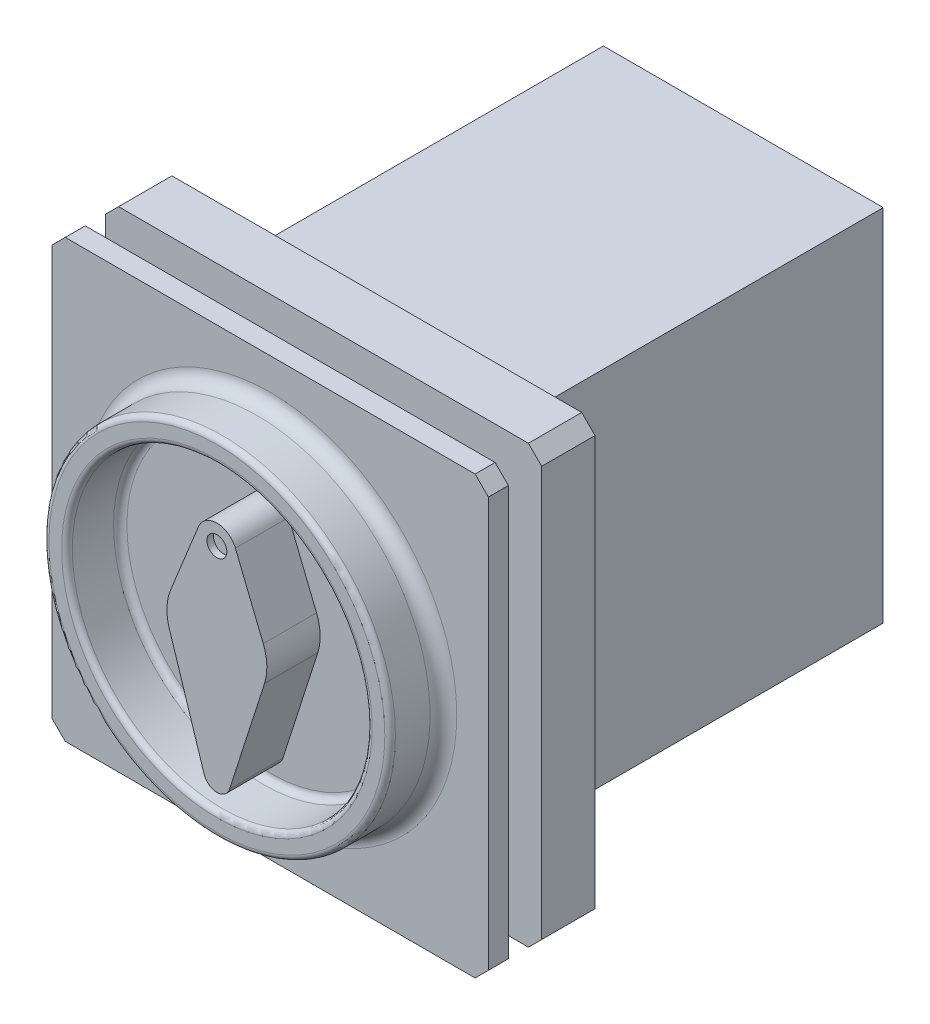
from build123d import *

# Parameters (mm, degrees)
SKETCH_1_W             = 42
SKETCH_1_H             = 54
EXTRUDE_1_DEPTH        = 55
SKETCH_5_W             = 65.5
SKETCH_5_H             = 65.5
EXTRUDE_3_DEPTH        = 8
SKETCH_6_R             = 10
EXTRUDE_4_DEPTH        = 5
HOLE_WIZARD_M4_1_D     = 3.3
HOLE_WIZARD_M4_1_DEPTH = 11.5
HOLE_WIZARD_M4_1_TIP   = 0.991420021
CHAMFER_1_SIZE         = 2
SKETCH_9_W             = 65.5
SKETCH_9_H             = 65.5
EXTRUDE_5_DEPTH        = 3
SKETCH_10_R            = 26
SKETCH_10_R_2          = 22.5
EXTRUDE_6_DEPTH        = 8
EXTRUDE_7_DEPTH        = 8
FILLET_1_R             = 2
FILLET_2_R             = 1
FILLET_3_R             = 0.8
SKETCH_12_R            = 1.5
CUT_EXTRUDE_1_DEPTH    = 1
CHAMFER_2_SIZE         = 2


with BuildPart() as part:
    # 草图1 → 凸台-拉伸1 (new body)
    with BuildSketch(Plane.XY):
        Rectangle(SKETCH_1_W, SKETCH_1_H)
    extrude(amount=EXTRUDE_1_DEPTH)

    # 草图5 → 凸台-拉伸3 (add)
    with BuildSketch(Plane.XY.offset(55)):
        Rectangle(SKETCH_5_W, SKETCH_5_H)
    extrude(amount=EXTRUDE_3_DEPTH)

    # 草图6 → 凸台-拉伸4 (add)
    with BuildSketch(Plane.XY.offset(63)):
        with Locations(Location((0, 0, 0), (0, 0, 180))):
            Circle(SKETCH_6_R)
    extrude(amount=EXTRUDE_4_DEPTH)

    # M4 螺纹孔1
    with Locations(Plane.XY.offset(63)):
        with Locations((-24, 24), (24, 24), (24, -24), (-24, -24)):
            Hole(HOLE_WIZARD_M4_1_D / 2, depth=HOLE_WIZARD_M4_1_DEPTH)
            with Locations((0, 0, -(HOLE_WIZARD_M4_1_DEPTH + HOLE_WIZARD_M4_1_TIP / 2))):  # 118° drill point
                Cone(0, HOLE_WIZARD_M4_1_D / 2, HOLE_WIZARD_M4_1_TIP, mode=Mode.SUBTRACT)

    # 倒角1
    chamfer_1_edges = [part.edges().sort_by_distance(p)[0] for p in [
        (32.75, -32.75, 59),
        (32.75, 32.75, 59),
        (-32.75, 32.75, 59),
        (-32.75, -32.75, 59),
    ]]
    chamfer(chamfer_1_edges, length=CHAMFER_1_SIZE)

    # 草图9 → 凸台-拉伸5 (add)
    with BuildSketch(Plane.XY.offset(68)):
        Rectangle(SKETCH_9_W, SKETCH_9_H)
    extrude(amount=EXTRUDE_5_DEPTH)

    # 草图10 → 凸台-拉伸6 (add)
    with BuildSketch(Plane.XY.offset(71)):
        with Locations(Location((0, 0, 0), (0, 0, 180))):
            Circle(SKETCH_10_R)
        Circle(SKETCH_10_R_2, mode=Mode.SUBTRACT)
    extrude(amount=EXTRUDE_6_DEPTH)

    # 草图11 → 凸台-拉伸7 (add)
    with BuildSketch(Plane.XY.offset(71)):
        with BuildLine():
            Line((2.781074433, 13.125), (6.952686082, 2.8125))
            ThreePointArc((6.952686082, 2.8125), (7.494884169, 0.276968033), (7.141306875, -2.291666667))
            Line((7.141306875, -2.291666667), (1.9043485, -18.611111111))
            ThreePointArc((1.9043485, -18.611111111), (0, -20), (-1.9043485, -18.611111111))
            Line((-1.9043485, -18.611111111), (-7.141306875, -2.291666667))
            ThreePointArc((-7.141306875, -2.291666667), (-7.494884169, 0.276968033), (-6.952686082, 2.8125))
            Line((-6.952686082, 2.8125), (-2.781074433, 13.125))
            ThreePointArc((-2.781074433, 13.125), (0, 15), (2.781074433, 13.125))
        make_face()
    extrude(amount=EXTRUDE_7_DEPTH)

    # 圆角1
    fillet_1_edges = [part.edges().sort_by_distance(p)[0] for p in [
        (26, 0, 71),
    ]]
    fillet(fillet_1_edges, radius=FILLET_1_R)

    # 圆角2
    fillet_2_edges = [part.edges().sort_by_distance(p)[0] for p in [
        (-22.5, 0, 71),
    ]]
    fillet(fillet_2_edges, radius=FILLET_2_R)

    # 圆角3
    fillet_3_edges = [part.edges().sort_by_distance(p)[0] for p in [
        (26, 0, 79),
        (-22.5, 0, 79),
    ]]
    fillet(fillet_3_edges, radius=FILLET_3_R)

    # 草图12 → 切除-拉伸1 (cut)
    with BuildSketch(Plane.XY.offset(79)):
        with Locations((0, 12)):
            Circle(SKETCH_12_R)
    extrude(amount=-CUT_EXTRUDE_1_DEPTH, mode=Mode.SUBTRACT)

    # 倒角2
    chamfer_2_edges = [part.edges().sort_by_distance(p)[0] for p in [
        (32.75, -32.75, 69.5),
        (32.75, 32.75, 69.5),
        (-32.75, 32.75, 69.5),
        (-32.75, -32.75, 69.5),
    ]]
    chamfer(chamfer_2_edges, length=CHAMFER_2_SIZE)


solid = part.part
